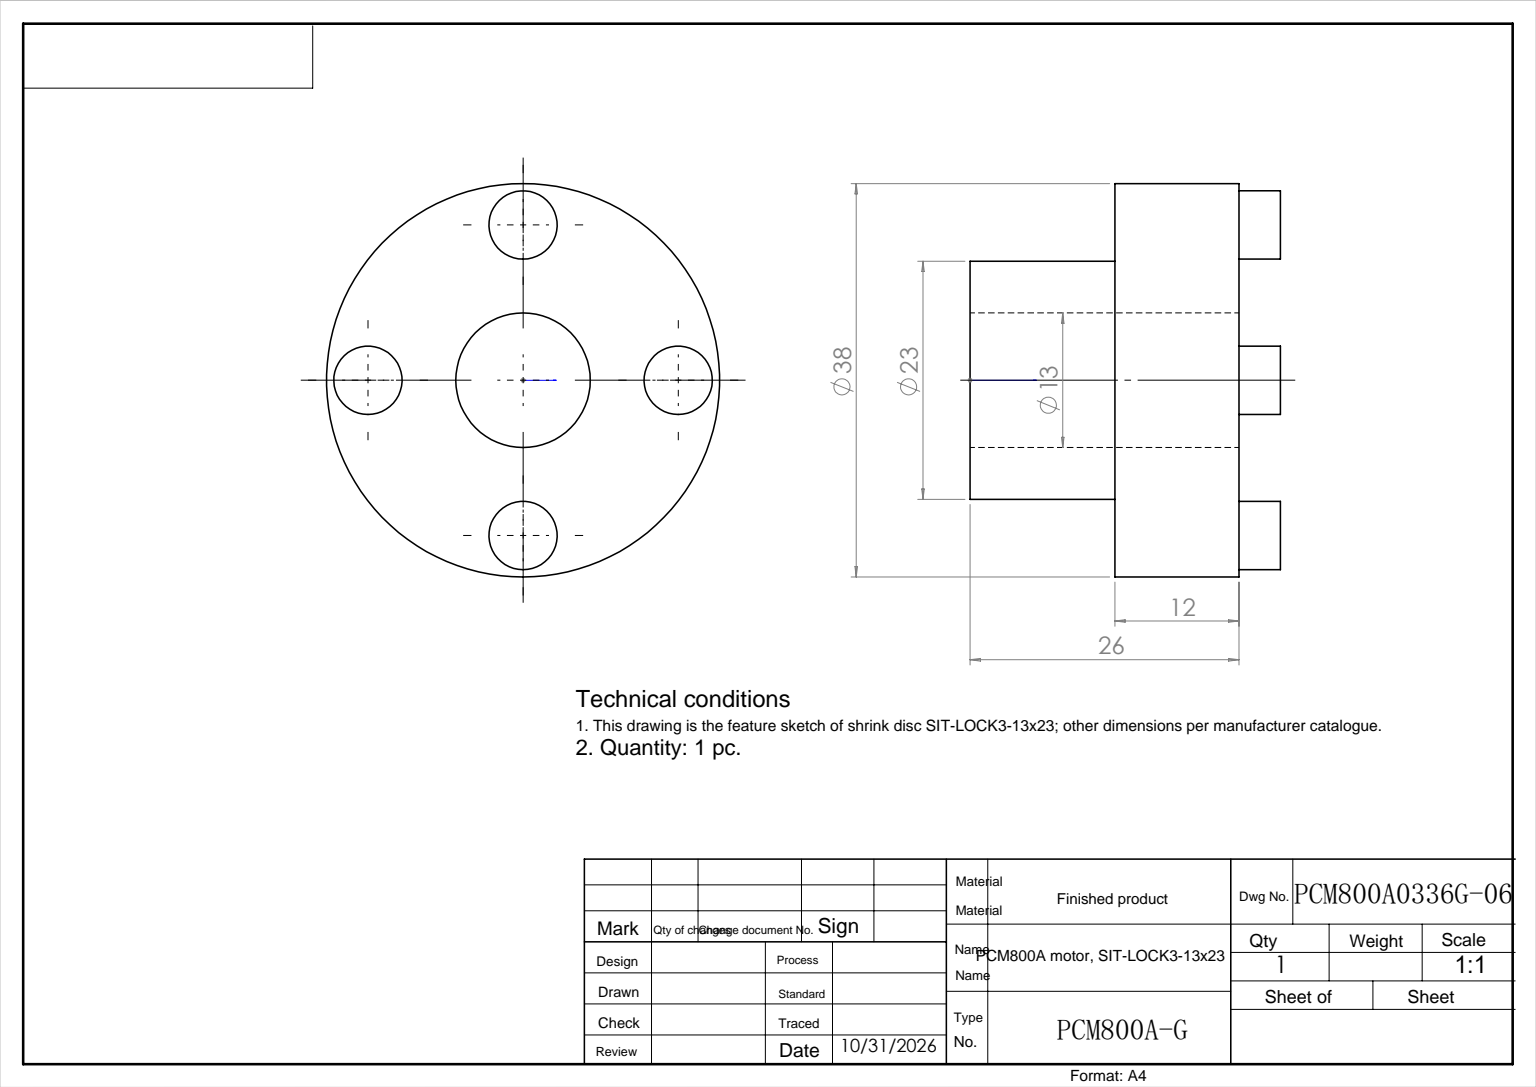
SolidWorks part; units mm, degrees
ref_plane "前视基准面" through (0, 0, 0) normal (0, 0, 1) x (1, 0, 0)
ref_plane "上视基准面" through (0, 0, 0) normal (0, 1, 0) x (1, 0, 0)
ref_plane "右视基准面" through (0, 0, 0) normal (1, 0, 0) x (0, 0, -1)
sketch "草图1" plane through (0, 0, 0) normal (0, 1, 0) x (1, 0, 0)
  circle A0 centre (0, 0) radius 6.5
  circle A1 centre (0, 0) radius 11.5
extrude "拉伸1" add sketch "草图1" along normal blind 14
sketch "草图2" plane through (0, 14, 0) normal (0, 1, 0) x (-1, 0, 0)
  circle A0 centre (0, 0) radius 6.5
  circle A1 centre (0, 0) radius 19
extrude "拉伸2" add sketch "草图2" along normal blind 12
sketch "草图3" plane through (0, 26, 0) normal (0, 1, 0) x (-1, 0, 0)
  circle A0 centre (0, 0) radius 15 construction
  circle A1 centre (-15, 0) radius 3.3
  circle A2 centre (0, -15) radius 3.3
  circle A3 centre (0, 15) radius 3.3
  circle A4 centre (15, 0) radius 3.3
extrude "拉伸3" add sketch "草图3" along normal blind 4
